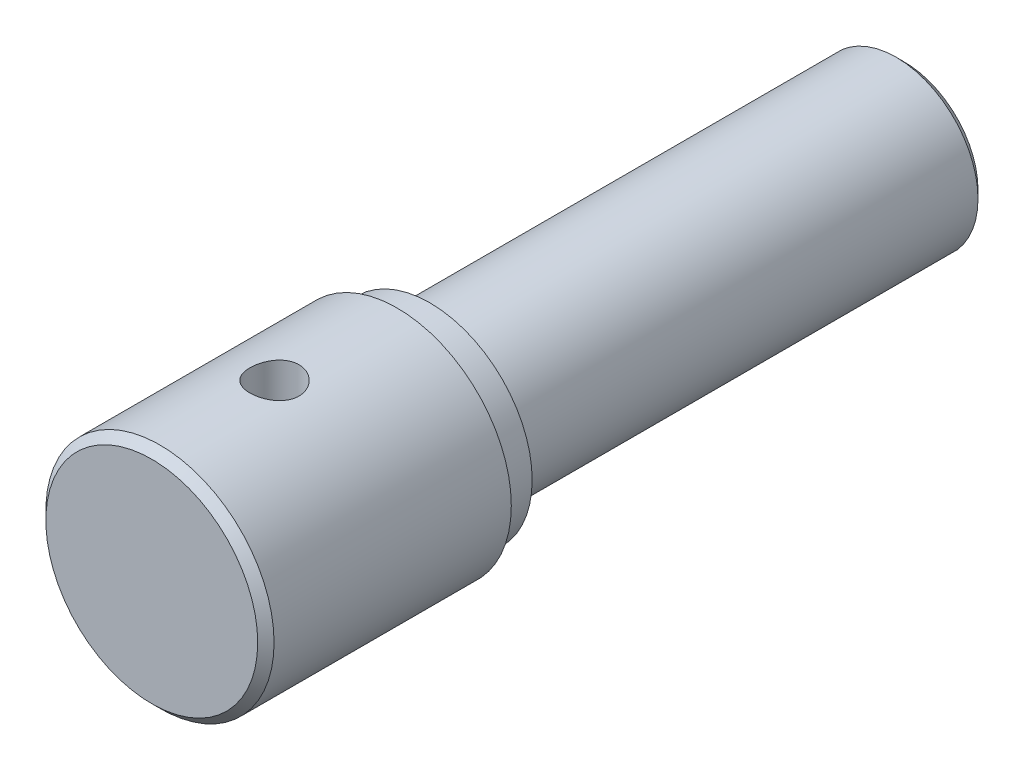
from build123d import *

# Parameters (mm, degrees)
SKETCH_1_R          = 10
EXTRUDE_1_DEPTH     = 58
SKETCH_2_R          = 12.5
EXTRUDE_2_DEPTH     = 4
SKETCH_3_R          = 13.95
EXTRUDE_3_DEPTH     = 30
CHAMFER_1_SIZE      = 1
FILLET_1_R          = 0.5
SKETCH_4_R          = 3
CUT_EXTRUDE_1_DEPTH = 15


with BuildPart() as part:
    # 草图1 → 凸台-拉伸1 (new body)
    with BuildSketch(Plane.XY):
        with Locations(Location((0, 0, 0), (0, 0, 180))):
            Circle(SKETCH_1_R)
    extrude(amount=EXTRUDE_1_DEPTH)

    # 草图2 → 凸台-拉伸2 (add)
    with BuildSketch(Plane.XY.offset(58)):
        Circle(SKETCH_2_R)
    extrude(amount=EXTRUDE_2_DEPTH)

    # 草图3 → 凸台-拉伸3 (add)
    with BuildSketch(Plane.XY.offset(62)):
        Circle(SKETCH_3_R)
    extrude(amount=EXTRUDE_3_DEPTH)

    # 倒角1
    chamfer_1_edges = [part.edges().sort_by_distance(p)[0] for p in [
        (-13.95, 0, 92),
        (10, 0, 0),
    ]]
    chamfer(chamfer_1_edges, length=CHAMFER_1_SIZE)

    # 圆角1
    fillet_1_edges = [part.edges().sort_by_distance(p)[0] for p in [
        (10, 0, 58),
    ]]
    fillet(fillet_1_edges, radius=FILLET_1_R)

    # 草图4 → 切除-拉伸1 (cut, symmetric)
    with BuildSketch(Plane(origin=(0, 0, 0), x_dir=(1, 0, 0), z_dir=(0, 1, 0))):
        with Locations(Location((0, -77, 0), (0, 0, 270))):
            Circle(SKETCH_4_R)
    extrude(amount=CUT_EXTRUDE_1_DEPTH, both=True, mode=Mode.SUBTRACT)


solid = part.part
